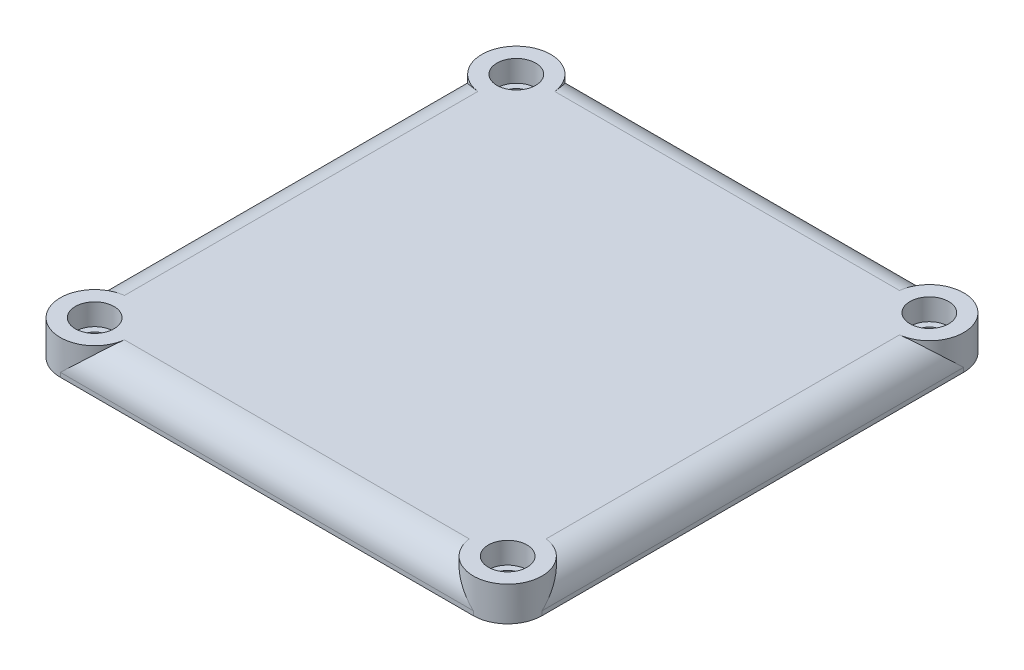
SolidWorks part; units mm, degrees
ref_plane "Front Plane" through (0, 0, 0) normal (0, 0, 1) x (1, 0, 0)
ref_plane "Top Plane" through (0, 0, 0) normal (0, 1, 0) x (1, 0, 0)
ref_plane "Right Plane" through (0, 0, 0) normal (1, 0, 0) x (0, 0, -1)
other "Configuration Table"
sketch "Sketch1" plane through (0, 0, 0) normal (0, 1, 0) x (1, 0, 0)
  line L1 (-48, -57) -> (48, -57)
  line L2 (-56, -49) -> (-56, 49)
  line L3 (-48, 57) -> (48, 57)
  line L4 (56, -49) -> (56, 49)
  line L5 (-56, -57) -> (56, 57) construction
  line L6 (-56, 57) -> (56, -57) construction
  arc A0 (48, -57) -> (56, -49) centre (48, -49) ccw
  arc A1 (-56, 49) -> (-48, 57) centre (-48, 49) cw
  arc A2 (-48, -57) -> (-56, -49) centre (-48, -49) cw
  arc A3 (48, 57) -> (56, 49) centre (48, 49) cw
  point P0 (0, 0)
  dimension "D3" = 8
  dimension "D1" = 114
  dimension "D2" = 112
extrude "Boss-Extrude1" add sketch "Sketch1" along normal blind 8
fillet "Fillet4" radius 7 8 edges at (0, 8, 57) (-53.6569, 8, 54.6569) (-56, 8, 0) (-53.6569, 8, -54.6569) (0, 8, -57) (53.6569, 8, -54.6569) (56, 8, 0) (53.6569, 8, 54.6569)
sketch "Sketch2" plane through (0, 0, 0) normal (0, -1, 0) x (-1, 0, 0)
  circle A0 centre (48, -49) radius 8
  circle A1 centre (-48, -49) radius 8
  circle A2 centre (-48, 49) radius 8
  circle A3 centre (48, 49) radius 8
  dimension "D1" = 16
  dimension "D2" = 16
  dimension "D3" = 16
  dimension "D4" = 16
extrude "Boss-Extrude2" add sketch "Sketch2" against normal blind 8
sketch "Sketch6" plane through (0, 0, 0) normal (0, -1, 0) x (-1, 0, 0)
  line L0 (-56, -49) -> (-56, 49) construction
  line L1 (49, -49) -> (-49, -49)
  line L2 (49, -49) -> (49, 49)
  line L3 (49, 49) -> (-49, 49)
  line L4 (-49, -49) -> (-49, 49)
  line L5 (49, -49) -> (-49, 49) construction
  line L6 (49, 49) -> (-49, -49) construction
  line L7 (51, 49) -> (49, 49) construction
  line L9 (0, -66.2877) -> (0, 0) construction
  line L10 (0, 0) -> (92.6706, 0) construction
  circle A2 centre (48, 49) radius 8
  circle A3 centre (48, -49) radius 8
  circle A4 centre (-48, 49) radius 8
  circle A5 centre (-48, -49) radius 8
  point P0 (0, 0)
  dimension "D3" = 16
  dimension "D1" = 7
  dimension "D2" = 98
extrude "Cut-Extrude1" cut sketch "Sketch6" against normal blind 3 contours A5 L1 A3 L2 A2 L3 A4 L4
fillet "Fillet3" radius 2 8 edges at (49, 3, 0) (42.7085, 3, -43) (0, 3, -49) (-42.7085, 3, -43) (-49, 3, 0) (-42.7085, 3, 43) (0, 3, 49) (42.7085, 3, 43)
hole_wizard "Hole2" positions "Sketch7" profile "Sketch8" legacy
sketch "Sketch7" plane through (0, 8, 0) normal (0, 1, 0) x (1, 0, 0)
  point P0 (-48, 49)
  point P3 (48, 49)
  point P6 (48, -49.8602)
  point P8 (-48, -49)
  point P12 (48, -49)
sketch "Sketch8" plane through (-48, 8, -49) normal (1, 0, 0) x (0, 0, 1)
  line L0 (0, 0) -> (0, 100)
  line L1 (0, 100) -> (3, 100)
  line L2 (3, 100) -> (3, 5)
  line L3 (3, 5) -> (4.5, 5)
  line L4 (4.5, 5) -> (4.5, 0)
  line L5 (4.5, 0) -> (0, 0)
  line L6 (0, 110) -> (0, -10) construction
  dimension "直径" = 6
  dimension "深度" = 100
  dimension "柱坑直径" = 9
  dimension "柱坑深度" = 5
